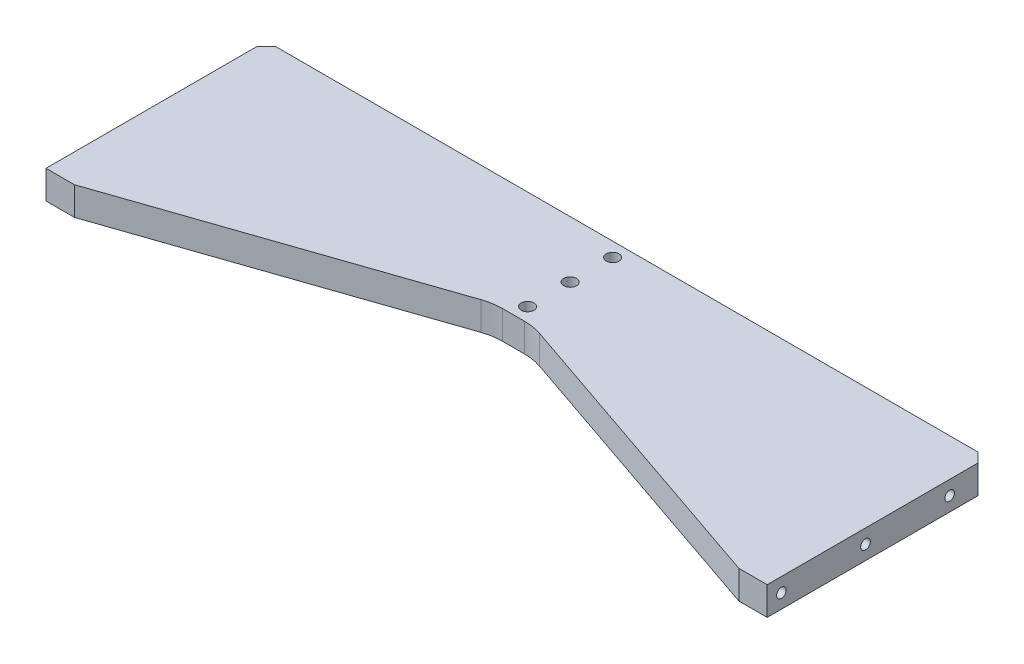
SolidWorks part; units mm, degrees
material "普通碳钢"
ref_plane "前视基准面" through (0, 0, 0) normal (0, 0, 1) x (1, 0, 0)
ref_plane "上视基准面" through (0, 0, 0) normal (0, 1, 0) x (1, 0, 0)
ref_plane "右视基准面" through (0, 0, 0) normal (1, 0, 0) x (0, 0, -1)
sketch "草图1" plane through (0, 0, 0) normal (0, 1, 0) x (1, 0, 0)
  line L1 (-381.5, -116.5) -> (381.5, -116.5)
  line L2 (-381.5, -116.5) -> (-381.5, 116.5)
  line L3 (-381.5, 116.5) -> (381.5, 116.5)
  line L4 (381.5, -116.5) -> (381.5, 116.5)
  line L5 (-381.5, -116.5) -> (381.5, 116.5) construction
  line L6 (-381.5, 116.5) -> (381.5, -116.5) construction
  point P0 (0, 0)
  dimension "D1" = 763
  dimension "D2" = 233
extrude "凸台-拉伸1" add sketch "草图1" along normal blind 30
chamfer "倒角1" distance 10 angle 45 2 edges at (381.5, 15, -116.5) (-381.5, 15, -116.5)
sketch "草图2" plane through (0, 30, 0) normal (0, 1, 0) x (1, 0, 0)
  line L0 (-351.5, -116.5) -> (-21.5, -3.5)
  line L1 (-381.5, -116.5) -> (381.5, -116.5) construction
  line L2 (-21.5, -3.5) -> (21.5, -3.5)
  line L3 (21.5, -3.5) -> (351.5, -116.5)
  line L4 (-381.5, 106.5) -> (-381.5, -116.5) construction
  line L5 (381.5, -116.5) -> (381.5, 106.5) construction
  dimension "D1" = 360
  dimension "D2" = 360
  dimension "D3" = 30
  dimension "D4" = 30
  dimension "D5" = 113
extrude "切除-拉伸1" cut sketch "草图2" against normal blind 30 and the other way through all flip side to cut
fillet "圆角1" radius 60 2 edges at (21.5, 15, 3.5) (-21.5, 15, 3.5)
hole_wizard "打孔尺寸(%根据)内六角圆柱头螺钉的类型1" positions "草图3" profile "草图4" counterbore size "M12" standard "GB" end condition through all
sketch "草图3" plane through (0, 0, 0) normal (0, -1, 0) x (-1, 0, 0)
  point P0 (0, 11.5)
  point P2 (0, 56.5)
  point P4 (0, 101.5)
  dimension "D1" = 351.5
  dimension "D2" = 128
  dimension "D3" = 173
  dimension "D4" = 218
sketch "草图4" plane through (0, 0, -11.5) normal (1, 0, 0) x (0, 0, -1)
  line L0 (0, 0) -> (0, 30)
  line L1 (0, 30) -> (6.75, 30)
  line L3 (6.75, 30) -> (6.75, 13)
  line L4 (6.75, 13) -> (10, 13)
  line L5 (10, 13) -> (10, 0)
  line L7 (10, 0) -> (0, 0)
  line L11 (0, -6.35) -> (0, 107.95) construction
  dimension "通孔孔直径" = 13.5
  dimension "通孔孔深度" = 30
  dimension "柱形沉头孔直径" = 20
  dimension "柱形沉头孔深度" = 13
hole_wizard "M12 螺纹孔1" positions "草图5" profile "草图6" tap size "M12" standard "GB"
sketch "草图5" plane through (0, 0, -116.5) normal (0, 0, -1) x (-1, 0, 0)
  line L0 (-381.5, 0) -> (-381.5, 30) construction
  line L1 (381.5, 30) -> (381.5, 0) construction
  line L2 (351.5, 15) -> (251.0714, 15) construction
  line L3 (251.0714, 15) -> (150.6429, 15) construction
  line L4 (150.6429, 15) -> (50.2143, 15) construction
  line L5 (50.2143, 15) -> (-50.2143, 15) construction
  line L6 (-50.2143, 15) -> (-150.6429, 15) construction
  line L7 (-150.6429, 15) -> (-251.0714, 15) construction
  line L8 (-251.0714, 15) -> (-351.5, 15) construction
  point P0 (351.5, 15)
  point P2 (251.0714, 15)
  point P4 (150.6429, 15)
  point P6 (50.2143, 15)
  point P8 (-50.2143, 15)
  point P10 (-150.6429, 15)
  point P12 (-251.0714, 15)
  point P14 (-351.5, 15)
  point P25 (-381.5, 15)
  dimension "D1" = 30
  dimension "D2" = 30
sketch "草图6" plane through (-351.5, 15, -116.5) normal (1, 0, 0) x (0, 1, 0)
  line L0 (0, 0) -> (0, 32.3144)
  line L1 (0, 32.3144) -> (5.1, 29.25)
  line L2 (5.1, 29.25) -> (5.1, 0)
  line L5 (5.1, 0) -> (0, 0)
  line L10 (0, 32.3144) -> (-5.1, 29.25) construction
  line L11 (0, -6.35) -> (0, 107.95) construction
  dimension "螺纹孔钻头直径" = 10.2
  dimension "螺纹孔钻头深度" = 29.25
  dimension "导头角度" = 118
cosmetic thread "孔螺蚊线1" parameters "D1"=24, "D2"=12
cosmetic thread "孔螺蚊线2" parameters "D1"=24, "D2"=12
cosmetic thread "孔螺蚊线3" parameters "D1"=24, "D2"=12
cosmetic thread "孔螺蚊线4" parameters "D1"=24, "D2"=12
cosmetic thread "孔螺蚊线5" parameters "D1"=24, "D2"=12
cosmetic thread "孔螺蚊线6" parameters "D1"=24, "D2"=12
cosmetic thread "孔螺蚊线7" parameters "D1"=24, "D2"=12
cosmetic thread "孔螺蚊线8" parameters "D1"=24, "D2"=12
hole_wizard "M12 螺纹孔2" positions "草图7" profile "草图8" tap size "M12" standard "GB"
sketch "草图7" plane through (-381.5, 0, 0) normal (-1, 0, 0) x (0, 0, 1)
  line L0 (-116.5, 0) -> (-116.5, 30) construction
  line L1 (116.5, 30) -> (116.5, 0) construction
  line L2 (101.5, 15) -> (12.5, 15) construction
  line L3 (12.5, 15) -> (-76.5, 15) construction
  point P0 (-76.5, 15)
  point P2 (12.5, 15)
  point P4 (101.5, 15)
  point P11 (116.5, 15)
  dimension "D1" = 40
  dimension "D2" = 15
sketch "草图8" plane through (-381.5, 15, -76.5) normal (0, 1, 0) x (0, 0, 1)
  line L0 (0, 0) -> (0, 32.3144)
  line L1 (0, 32.3144) -> (5.1, 29.25)
  line L2 (5.1, 29.25) -> (5.1, 0)
  line L5 (5.1, 0) -> (0, 0)
  line L10 (0, 32.3144) -> (-5.1, 29.25) construction
  line L11 (0, -6.35) -> (0, 107.95) construction
  dimension "螺纹孔钻头直径" = 10.2
  dimension "螺纹孔钻头深度" = 29.25
  dimension "导头角度" = 118
cosmetic thread "孔螺蚊线9" parameters "D1"=24, "D2"=12
cosmetic thread "孔螺蚊线10" parameters "D1"=24, "D2"=12
cosmetic thread "孔螺蚊线11" parameters "D1"=24, "D2"=12
hole_wizard "M12 螺纹孔3" positions "草图9" profile "草图10" tap size "M12" standard "GB"
sketch "草图9" plane through (381.5, 0, 0) normal (1, 0, 0) x (0, 0, -1)
  line L0 (-116.5, 0) -> (106.5, 0) construction
  point P0 (76.5, 15)
  point P2 (-12.5, 15)
  point P4 (-101.5, 15)
  dimension "D1" = 15
  dimension "D2" = 104
  dimension "D3" = 193
  dimension "D4" = 15
sketch "草图10" plane through (381.5, 15, -76.5) normal (0, 1, 0) x (0, 0, -1)
  line L0 (0, 0) -> (0, 32.3144)
  line L1 (0, 32.3144) -> (5.1, 29.25)
  line L2 (5.1, 29.25) -> (5.1, 0)
  line L5 (5.1, 0) -> (0, 0)
  line L10 (0, 32.3144) -> (-5.1, 29.25) construction
  line L11 (0, -6.35) -> (0, 107.95) construction
  dimension "螺纹孔钻头直径" = 10.2
  dimension "螺纹孔钻头深度" = 29.25
  dimension "导头角度" = 118
cosmetic thread "孔螺蚊线12" parameters "D1"=24, "D2"=12
cosmetic thread "孔螺蚊线13" parameters "D1"=24, "D2"=12
cosmetic thread "孔螺蚊线14" parameters "D1"=24, "D2"=12
